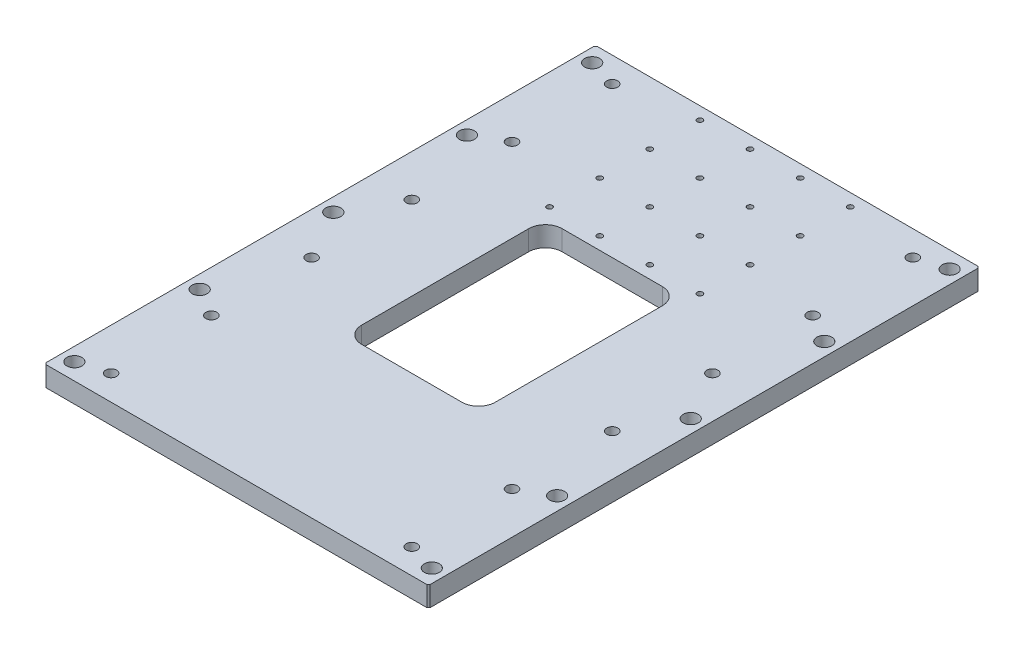
from build123d import *

# Parameters (mm, degrees)
SKETCH_1_W                = 230
SKETCH_1_H                = 330
EXTRUDE_1_DEPTH           = 6
HOLE_WIZARD_M8_1_D        = 9
CHAMFER_1_SIZE            = 1
HOLE_WIZARD_1_D           = 6.6
HOLE_WIZARD_1_CBORE_D     = 11
HOLE_WIZARD_1_CBORE_DEPTH = 6.8
SKETCH_6_W                = 80
SKETCH_6_H                = 120
CUT_EXTRUDE_1_DEPTH       = 202.479527496
FILLET_1_R                = 10
HOLE_WIZARD_M4_1_D        = 3.3


with BuildPart() as part:
    # 草图1 → 凸台-拉伸1 (new, symmetric)
    with BuildSketch(Plane(origin=(0, 0, 0), x_dir=(1, 0, 0), z_dir=(0, 1, 0))):
        Rectangle(SKETCH_1_W, SKETCH_1_H)
    extrude(amount=EXTRUDE_1_DEPTH, both=True)

    # M8 间隙孔1 (through all)
    with Locations(Plane(origin=(0, 6, 0), x_dir=(1, 0, 0), z_dir=(0, 1, 0))):
        with Locations((-107, 155), (-107, 80), (107, 80), (107, 155), (-107, 0), (-107, -155), (-107, -80), (107, -80), (107, -155), (107, 0)):
            Hole(HOLE_WIZARD_M8_1_D / 2)

    # 倒角1
    chamfer_1_edges = [part.edges().sort_by_distance(p)[0] for p in [
        (115, 0, 165),
        (-115, 0, 165),
        (-115, 0, -165),
        (115, 0, -165),
    ]]
    chamfer(chamfer_1_edges, length=CHAMFER_1_SIZE)

    # 打孔尺寸(%根据)内六角圆柱头螺钉的类型1 (through all)
    with Locations(Plane(origin=(0, -6, 0), x_dir=(-1, 0, 0), z_dir=(0, -1, 0))):
        with Locations((90, -150), (-90, -150), (90, -90), (-90, -90), (90, -30), (-90, -30), (90, 30), (-90, 30), (90, 90), (-90, 90), (90, 150), (-90, 150)):
            CounterBoreHole(HOLE_WIZARD_1_D / 2, HOLE_WIZARD_1_CBORE_D / 2, HOLE_WIZARD_1_CBORE_DEPTH)

    # 草图6 → 切除-拉伸1 (cut, through all)
    with BuildSketch(Plane(origin=(0, 6, 0), x_dir=(1, 0, 0), z_dir=(0, 1, 0))):
        Rectangle(SKETCH_6_W, SKETCH_6_H)
    extrude(amount=-CUT_EXTRUDE_1_DEPTH, mode=Mode.SUBTRACT)

    # 圆角1
    fillet_1_edges = [part.edges().sort_by_distance(p)[0] for p in [
        (40, 0, -60),
        (40, 0, 60),
        (-40, 0, 60),
        (-40, 0, -60),
    ]]
    fillet(fillet_1_edges, radius=FILLET_1_R)

    # M4 螺纹孔1 (through all)
    with Locations(Plane(origin=(0, 6, 0), x_dir=(1, 0, 0), z_dir=(0, 1, 0))):
        with Locations((-45, 67.5), (-45, 157.5), (-15, 157.5), (15, 157.5), (45, 157.5), (-15, 127.5), (15, 127.5), (45, 127.5), (-15, 97.5), (15, 97.5), (45, 97.5), (-15, 67.5), (15, 67.5), (45, 67.5), (-45, 127.5), (-45, 97.5)):
            Hole(HOLE_WIZARD_M4_1_D / 2)


solid = part.part
